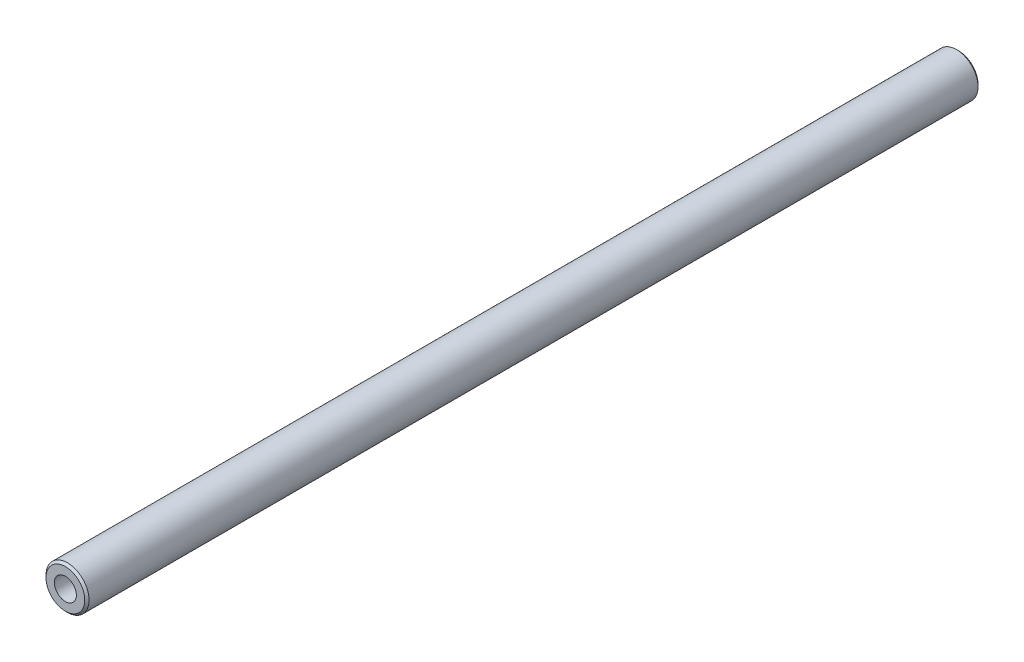
from build123d import *

# Parameters (mm, degrees)
HOLE_WIZARD_M12_5_D     = 10.2
HOLE_WIZARD_M12_5_DEPTH = 220
HOLE_WIZARD_M12_5_TIP   = 3.064389157
HOLE_WIZARD_M12_6_D     = 10.2
HOLE_WIZARD_M12_6_DEPTH = 220
HOLE_WIZARD_M12_6_TIP   = 3.064389157


with BuildPart() as part:
    # 草图1 → 旋转1 (revolve)
    with BuildSketch(Plane.XZ, mode=Mode.PRIVATE) as revolve_1_sk:
        Polygon((9, -207.5), (10, -206.5), (10, 206.5), (9, 207.5), (0, 207.5), (0, -207.5), align=None)
    revolve(revolve_1_sk.sketch.rotate(Axis((0, 0, 207.5), (0, 0, -1)), 180), axis=Axis((0, 0, 207.5), (0, 0, -1)))

    # M12 螺纹孔5
    with Locations(Plane(origin=(0, 0, -207.5), x_dir=(-1, 0, 0), z_dir=(0, 0, -1))):
        with Locations((0, 0)):
            Hole(HOLE_WIZARD_M12_5_D / 2, depth=HOLE_WIZARD_M12_5_DEPTH)
            with Locations((0, 0, -(HOLE_WIZARD_M12_5_DEPTH + HOLE_WIZARD_M12_5_TIP / 2))):  # 118° drill point
                Cone(0, HOLE_WIZARD_M12_5_D / 2, HOLE_WIZARD_M12_5_TIP, mode=Mode.SUBTRACT)

    # M12 螺纹孔6
    with Locations(Plane.XY.offset(207.5)):
        with Locations((0, 0)):
            Hole(HOLE_WIZARD_M12_6_D / 2, depth=HOLE_WIZARD_M12_6_DEPTH)
            with Locations((0, 0, -(HOLE_WIZARD_M12_6_DEPTH + HOLE_WIZARD_M12_6_TIP / 2))):  # 118° drill point
                Cone(0, HOLE_WIZARD_M12_6_D / 2, HOLE_WIZARD_M12_6_TIP, mode=Mode.SUBTRACT)


solid = part.part
